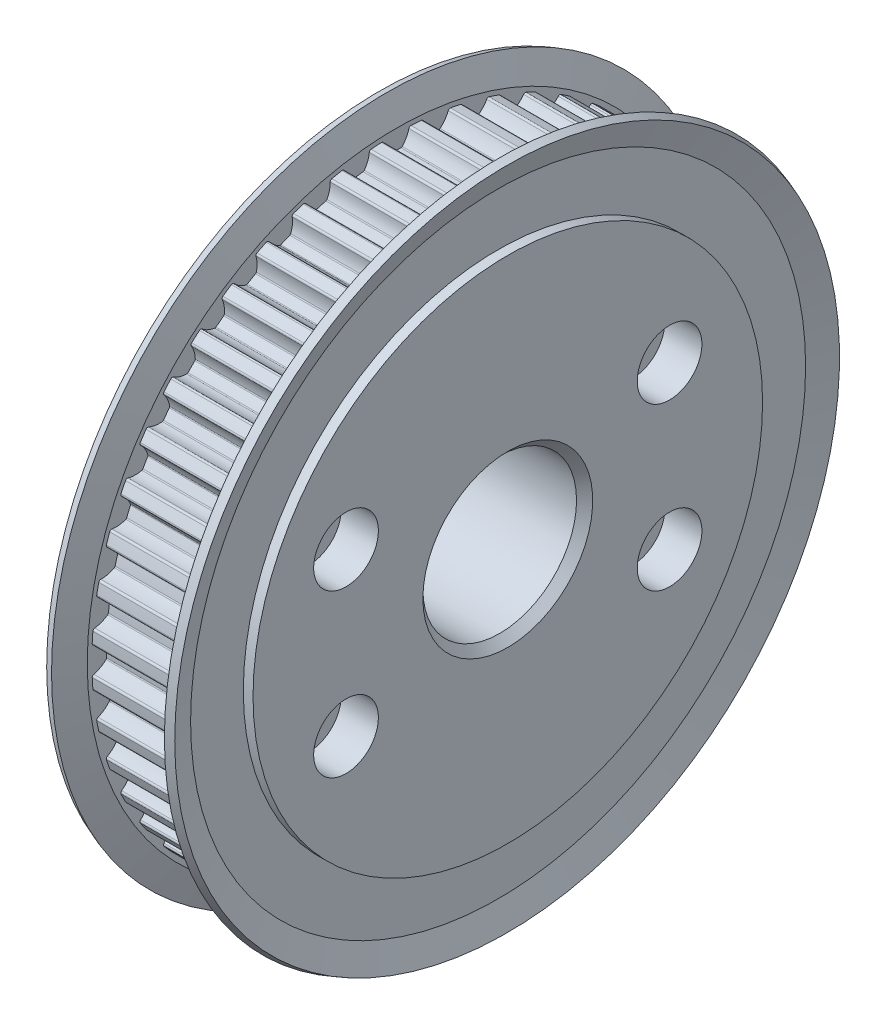
from build123d import *

# Parameters (mm, degrees)
SKETCH2_W                                            = 12
SKETCH2_H                                            = 30
SKETCH3_W                                            = 152.78
SKETCH3_H                                            = 152.78
CUT_EXTRUDE1_DEPTH                                   = 11.6
SKETCH4_R                                            = 9.5
CUT_EXTRUDE2_DEPTH                                   = 61.744199967
HOLE_SIZE_BY_SOCKET_HEAD_CAP_SCREW_TYPE1_D           = 4.5
HOLE_SIZE_BY_SOCKET_HEAD_CAP_SCREW_TYPE1_CBORE_D     = 8
HOLE_SIZE_BY_SOCKET_HEAD_CAP_SCREW_TYPE1_CBORE_DEPTH = 4.6
CHAMFER1_SIZE                                        = 1


with BuildPart() as part:
    # Sketch1 → Revolve1 (revolve)
    with BuildSketch(Plane.XY, mode=Mode.PRIVATE) as revolve1_sk:
        Polygon((0, 31.5), (0, 7.7), (0.2, 7.5), (27.8, 7.5), (28, 7.7), (28, 28.8), (27.8, 29), (16, 29), (16, 31.5), (14.8, 31.5), (14.8, 38.019075537), (15.916664119, 41.094554632), (14.97670473, 41.435840945), (13.8, 38.195), (2.2, 38.195), (1.02329527, 41.435840945), (0.083335881, 41.094554632), (1.2, 38.019075537), (1.2, 31.5), align=None)
    revolve(revolve1_sk.sketch.rotate(Axis((28, 0, 0), (-1, 0, 0)), 270), axis=Axis((28, 0, 0), (-1, 0, 0)))

    # Sketch2 → Cut-Revolve1 (revolve, cut)
    with BuildSketch(Plane.XY, mode=Mode.PRIVATE) as cut_revolve1_sk:
        with Locations((22, 15)):
            Rectangle(SKETCH2_W, SKETCH2_H)
    revolve(cut_revolve1_sk.sketch.rotate(Axis((28, 0, 0), (-1, 0, 0)), 270), axis=Axis((28, 0, 0), (-1, 0, 0)), mode=Mode.SUBTRACT)

    # Sketch3 → Cut-Extrude1 (cut)
    with BuildSketch(Plane(origin=(2.2, 0, 0), x_dir=(0, 0, -1), z_dir=(1, 0, 0))):
        Rectangle(SKETCH3_W, SKETCH3_H)
        with BuildLine():
            ThreePointArc((-37.580722706, 1.824802974), (-37.530923747, 1.662553905), (-37.388992694, 1.569493317))
            ThreePointArc((-37.388992694, 1.569493317), (-36.576235091, 1.258482416), (-35.87221643, 0.746954873))
            ThreePointArc((-35.87221643, 0.746954873), (-35.825535624, 0.679315888), (-35.809997004, 0.598614703))
            ThreePointArc((-35.809997004, 0.598614703), (-35.815, -3.6e-08), (-35.809997003, -0.598614776))
            ThreePointArc((-35.809997003, -0.598614776), (-35.825535638, -0.679315922), (-35.87221643, -0.746954873))
            ThreePointArc((-35.87221643, -0.746954873), (-36.57623506, -1.258482399), (-37.388992626, -1.569493301))
            ThreePointArc((-37.388992626, -1.569493301), (-37.530923726, -1.662553877), (-37.580722706, -1.824802974))
            ThreePointArc((-37.580722706, -1.824802974), (-37.563928353, -2.14287464), (-37.544441987, -2.460792737))
            ThreePointArc((-37.544441987, -2.460792737), (-37.522265005, -2.778534482), (-37.497398997, -3.096077104))
            ThreePointArc((-37.497398997, -3.096077104), (-37.426848324, -3.25043804), (-37.273984668, -3.324176762))
            ThreePointArc((-37.273984668, -3.324176762), (-36.427585249, -3.526440767), (-35.662821821, -3.941699246))
            ThreePointArc((-35.662821821, -3.941699246), (-35.607711717, -4.002666503), (-35.581772413, -4.080649081))
            ThreePointArc((-35.581772413, -4.080649081), (-35.508597705, -4.67479561), (-35.425502607, -5.267636096))
            ThreePointArc((-35.425502607, -5.267636096), (-35.430374694, -5.349675031), (-35.467827471, -5.422828388))
            ThreePointArc((-35.467827471, -5.422828388), (-36.099055384, -6.021872596), (-36.864264626, -6.436308907))
            ThreePointArc((-36.864264626, -6.436308907), (-36.992834644, -6.547099062), (-37.02102983, -6.714460168))
            ThreePointArc((-37.02102983, -6.714460168), (-36.962862471, -7.027618583), (-36.902046175, -7.340273366))
            ThreePointArc((-36.902046175, -7.340273366), (-36.838585301, -7.652402109), (-36.772484396, -7.963982444))
            ThreePointArc((-36.772484396, -7.963982444), (-36.682389148, -8.10781409), (-36.521208429, -8.160969257))
            ThreePointArc((-36.521208429, -8.160969257), (-35.655649323, -8.251025572), (-34.843226443, -8.562909799))
            ThreePointArc((-34.843226443, -8.562909799), (-34.78062999, -8.61616216), (-34.744733831, -8.690091828))
            ThreePointArc((-34.744733831, -8.690091828), (-34.594633459, -9.269604136), (-34.43486804, -9.846526701))
            ThreePointArc((-34.43486804, -9.846526701), (-34.428990216, -9.928499717), (-34.456574149, -10.005915805))
            ThreePointArc((-34.456574149, -10.005915805), (-35.004210861, -10.682226883), (-35.708778839, -11.192997482))
            ThreePointArc((-35.708778839, -11.192997482), (-35.821787905, -11.319621568), (-35.827896869, -11.489231086))
            ThreePointArc((-35.827896869, -11.489231086), (-35.729351764, -11.792118024), (-35.628246122, -12.094159882))
            ThreePointArc((-35.628246122, -12.094159882), (-35.524587188, -12.395335014), (-35.418382391, -12.695621837))
            ThreePointArc((-35.418382391, -12.695621837), (-35.310284058, -12.826463233), (-35.143544035, -12.858125281))
            ThreePointArc((-35.143544035, -12.858125281), (-34.273635274, -12.83443305), (-33.427453801, -13.037606591))
            ThreePointArc((-33.427453801, -13.037606591), (-33.35844204, -13.082232894), (-33.313203221, -13.150844695))
            ThreePointArc((-33.313203221, -13.150844695), (-33.088745443, -13.705807164), (-32.855043333, -14.256940505))
            ThreePointArc((-32.855043333, -14.256940505), (-32.838516169, -14.337445021), (-32.855759291, -14.417799229))
            ThreePointArc((-32.855759291, -14.417799229), (-33.310434585, -15.159805306), (-33.942305944, -15.758170768))
            ThreePointArc((-33.942305944, -15.758170768), (-34.037820443, -15.89846221), (-34.021738659, -16.067418075))
            ThreePointArc((-34.021738659, -16.067418075), (-33.884501943, -16.354851056), (-33.7448369, -16.641111969))
            ThreePointArc((-33.7448369, -16.641111969), (-33.602753539, -16.926180301), (-33.458262043, -17.21003562))
            ThreePointArc((-33.458262043, -17.21003562), (-33.334010276, -17.325647987), (-33.164564009, -17.33527522))
            ThreePointArc((-33.164564009, -17.33527522), (-32.305189896, -17.198239802), (-31.439728155, -17.289226319))
            ThreePointArc((-31.439728155, -17.289226319), (-31.365481893, -17.324463001), (-31.311674459, -17.386582976))
            ThreePointArc((-31.311674459, -17.386582976), (-31.016699814, -17.907500038), (-30.713059726, -18.423414104))
            ThreePointArc((-30.713059726, -18.423414104), (-30.686166006, -18.501072665), (-30.692773282, -18.582990111))
            ThreePointArc((-30.692773282, -18.582990111), (-31.046707538, -19.377995258), (-31.595070785, -20.053717383))
            ThreePointArc((-31.595070785, -20.053717383), (-31.671456436, -20.205275756), (-31.633459069, -20.370687086))
            ThreePointArc((-31.633459069, -20.370687086), (-31.459878899, -20.637748052), (-31.284044163, -20.903330017))
            ThreePointArc((-31.284044163, -20.903330017), (-31.105967461, -21.167413949), (-30.925661556, -21.429980923))
            ThreePointArc((-30.925661556, -21.429980923), (-30.787382335, -21.5283861), (-30.618129095, -21.515813792))
            ThreePointArc((-30.618129095, -21.515813792), (-29.783993761, -21.267779902), (-28.914060045, -21.245022592))
            ThreePointArc((-28.914060045, -21.245022592), (-28.835849659, -21.270266737), (-28.774394272, -21.324831987))
            ThreePointArc((-28.774394272, -21.324831987), (-28.413949856, -21.802790615), (-28.045567152, -22.27465798))
            ThreePointArc((-28.045567152, -22.27465798), (-28.008767035, -22.348141826), (-28.004625413, -22.43022088))
            ThreePointArc((-28.004625413, -22.43022088), (-28.251762717, -23.264622338), (-28.707235205, -24.006139333))
            ThreePointArc((-28.707235205, -24.006139333), (-28.763185029, -24.166371431), (-28.703922223, -24.325407993))
            ThreePointArc((-28.703922223, -24.325407993), (-28.496968605, -24.567527457), (-28.287972756, -24.807886293))
            ThreePointArc((-28.287972756, -24.807886293), (-28.076949655, -25.046467277), (-27.863914425, -25.28325331))
            ThreePointArc((-27.863914425, -25.28325331), (-27.713973748, -25.362767557), (-27.547809509, -25.328210825))
            ThreePointArc((-27.547809509, -25.328210825), (-26.753185238, -24.973422391), (-25.89366435, -24.837310638))
            ThreePointArc((-25.89366435, -24.837310638), (-25.812828043, -24.852130312), (-25.744776221, -24.898207211))
            ThreePointArc((-25.744776221, -24.898207211), (-25.325029337, -25.325029399), (-24.898207148, -25.744776282))
            ThreePointArc((-24.898207148, -25.744776282), (-24.852130295, -25.812828084), (-24.837310638, -25.89366435))
            ThreePointArc((-24.837310638, -25.89366435), (-24.973422403, -26.75318528), (-25.328210871, -27.547809584))
            ThreePointArc((-25.328210871, -27.547809584), (-25.362767551, -27.713973791), (-25.28325331, -27.863914425))
            ThreePointArc((-25.28325331, -27.863914425), (-25.046467277, -28.076949655), (-24.807886293, -28.287972756))
            ThreePointArc((-24.807886293, -28.287972756), (-24.567527457, -28.496968605), (-24.325407993, -28.703922223))
            ThreePointArc((-24.325407993, -28.703922223), (-24.166371472, -28.763185028), (-24.006139396, -28.707235256))
            ThreePointArc((-24.006139396, -28.707235256), (-23.264622375, -28.251762734), (-22.43022088, -28.004625413))
            ThreePointArc((-22.43022088, -28.004625413), (-22.348141783, -28.008767047), (-22.274657911, -28.045567207))
            ThreePointArc((-22.274657911, -28.045567207), (-21.802790545, -28.413949909), (-21.324831916, -28.774394325))
            ThreePointArc((-21.324831916, -28.774394325), (-21.270266715, -28.835849698), (-21.245022592, -28.914060045))
            ThreePointArc((-21.245022592, -28.914060045), (-21.267779908, -29.783993804), (-21.515813827, -30.618129175))
            ThreePointArc((-21.515813827, -30.618129175), (-21.528386088, -30.787382376), (-21.429980923, -30.925661556))
            ThreePointArc((-21.429980923, -30.925661556), (-21.167413949, -31.105967461), (-20.903330017, -31.284044163))
            ThreePointArc((-20.903330017, -31.284044163), (-20.637748052, -31.459878899), (-20.370687086, -31.633459069))
            ThreePointArc((-20.370687086, -31.633459069), (-20.205275801, -31.671456442), (-20.053717445, -31.595070851))
            ThreePointArc((-20.053717445, -31.595070851), (-19.377995297, -31.046707562), (-18.582990111, -30.692773282))
            ThreePointArc((-18.582990111, -30.692773282), (-18.501072611, -30.686166013), (-18.423414012, -30.713059781))
            ThreePointArc((-18.423414012, -30.713059781), (-17.907499953, -31.016699863), (-17.386582899, -31.311674502))
            ThreePointArc((-17.386582899, -31.311674502), (-17.324462974, -31.365481928), (-17.289226319, -31.439728155))
            ThreePointArc((-17.289226319, -31.439728155), (-17.198239803, -32.305189937), (-17.335275243, -33.164564086))
            ThreePointArc((-17.335275243, -33.164564086), (-17.325647971, -33.334010313), (-17.21003562, -33.458262043))
            ThreePointArc((-17.21003562, -33.458262043), (-16.926180301, -33.602753539), (-16.64111197, -33.7448369))
            ThreePointArc((-16.64111197, -33.7448369), (-16.354851056, -33.884501943), (-16.067418075, -34.021738659))
            ThreePointArc((-16.067418075, -34.021738659), (-15.898462259, -34.037820456), (-15.758170827, -33.942306026))
            ThreePointArc((-15.758170827, -33.942306026), (-15.159805346, -33.310434617), (-14.417799229, -32.855759291))
            ThreePointArc((-14.417799229, -32.855759291), (-14.337444967, -32.838516169), (-14.256940407, -32.855043376))
            ThreePointArc((-14.256940407, -32.855043376), (-13.70580708, -33.088745478), (-13.150844627, -33.313203247))
            ThreePointArc((-13.150844627, -33.313203247), (-13.082232868, -33.358442066), (-13.037606591, -33.427453801))
            ThreePointArc((-13.037606591, -33.427453801), (-12.834433046, -34.273635313), (-12.858125293, -35.143544112))
            ThreePointArc((-12.858125293, -35.143544112), (-12.826463213, -35.310284091), (-12.695621837, -35.418382391))
            ThreePointArc((-12.695621837, -35.418382391), (-12.395335014, -35.524587188), (-12.094159882, -35.628246122))
            ThreePointArc((-12.094159882, -35.628246122), (-11.792118024, -35.729351765), (-11.489231086, -35.827896869))
            ThreePointArc((-11.489231086, -35.827896869), (-11.319621613, -35.821787923), (-11.192997529, -35.708778924))
            ThreePointArc((-11.192997529, -35.708778924), (-10.682226916, -35.004210896), (-10.005915805, -34.456574149))
            ThreePointArc((-10.005915805, -34.456574149), (-9.928499664, -34.428990208), (-9.846526598, -34.434868069))
            ThreePointArc((-9.846526598, -34.434868069), (-9.269604048, -34.594633483), (-8.690091757, -34.744733849))
            ThreePointArc((-8.690091757, -34.744733849), (-8.616162131, -34.780630012), (-8.562909799, -34.843226443))
            ThreePointArc((-8.562909799, -34.843226443), (-8.251025581, -35.655649286), (-8.160969255, -36.521208354))
            ThreePointArc((-8.160969255, -36.521208354), (-8.107814114, -36.682389119), (-7.963982444, -36.772484396))
            ThreePointArc((-7.963982444, -36.772484396), (-7.652402109, -36.838585301), (-7.340273366, -36.902046175))
            ThreePointArc((-7.340273366, -36.902046175), (-7.027618583, -36.962862471), (-6.714460168, -37.02102983))
            ThreePointArc((-6.714460168, -37.02102983), (-6.547099105, -36.992834668), (-6.436308941, -36.864264717))
            ThreePointArc((-6.436308941, -36.864264717), (-6.021872624, -36.099055423), (-5.422828388, -35.467827471))
            ThreePointArc((-5.422828388, -35.467827471), (-5.349674979, -35.43037468), (-5.267635989, -35.425502623))
            ThreePointArc((-5.267635989, -35.425502623), (-4.674795521, -35.508597717), (-4.080649009, -35.581772422))
            ThreePointArc((-4.080649009, -35.581772422), (-4.002666471, -35.607711735), (-3.941699246, -35.662821821))
            ThreePointArc((-3.941699246, -35.662821821), (-3.526440781, -36.427585215), (-3.32417677, -37.273984595))
            ThreePointArc((-3.32417677, -37.273984595), (-3.250438067, -37.426848298), (-3.096077104, -37.497398997))
            ThreePointArc((-3.096077104, -37.497398997), (-2.778534482, -37.522265005), (-2.460792737, -37.544441987))
            ThreePointArc((-2.460792737, -37.544441987), (-2.14287464, -37.563928353), (-1.824802974, -37.580722706))
            ThreePointArc((-1.824802974, -37.580722706), (-1.662553917, -37.530923757), (-1.569493325, -37.388992724))
            ThreePointArc((-1.569493325, -37.388992724), (-1.258482423, -36.576235105), (-0.746954873, -35.87221643))
            ThreePointArc((-0.746954873, -35.87221643), (-0.679315872, -35.825535618), (-0.598614668, -35.809997005))
            ThreePointArc((-0.598614668, -35.809997005), (5.4e-08, -35.815), (0.598614776, -35.809997003))
            ThreePointArc((0.598614776, -35.809997003), (0.679315922, -35.825535638), (0.746954873, -35.87221643))
            ThreePointArc((0.746954873, -35.87221643), (1.258482399, -36.57623506), (1.569493301, -37.388992626))
            ThreePointArc((1.569493301, -37.388992626), (1.662553877, -37.530923726), (1.824802974, -37.580722706))
            ThreePointArc((1.824802974, -37.580722706), (2.14287464, -37.563928353), (2.460792737, -37.544441987))
            ThreePointArc((2.460792737, -37.544441987), (2.778534482, -37.522265005), (3.096077104, -37.497398997))
            ThreePointArc((3.096077104, -37.497398997), (3.250438031, -37.426848333), (3.32417676, -37.273984695))
            ThreePointArc((3.32417676, -37.273984695), (3.526440763, -36.427585262), (3.941699246, -35.662821821))
            ThreePointArc((3.941699246, -35.662821821), (4.00266651, -35.607711713), (4.080649097, -35.581772412))
            ThreePointArc((4.080649097, -35.581772412), (4.674795618, -35.508597704), (5.267636096, -35.425502607))
            ThreePointArc((5.267636096, -35.425502607), (5.349675031, -35.430374694), (5.422828388, -35.467827471))
            ThreePointArc((5.422828388, -35.467827471), (6.021872596, -36.099055384), (6.436308907, -36.864264626))
            ThreePointArc((6.436308907, -36.864264626), (6.547099062, -36.992834644), (6.714460168, -37.02102983))
            ThreePointArc((6.714460168, -37.02102983), (7.027618583, -36.962862471), (7.340273366, -36.902046175))
            ThreePointArc((7.340273366, -36.902046175), (7.652402109, -36.838585301), (7.963982444, -36.772484396))
            ThreePointArc((7.963982444, -36.772484396), (8.107814082, -36.682389159), (8.160969258, -36.521208456))
            ThreePointArc((8.160969258, -36.521208456), (8.251025569, -35.655649336), (8.562909799, -34.843226443))
            ThreePointArc((8.562909799, -34.843226443), (8.616162166, -34.780629985), (8.690091843, -34.744733828))
            ThreePointArc((8.690091843, -34.744733828), (9.269604143, -34.594633457), (9.846526701, -34.43486804))
            ThreePointArc((9.846526701, -34.43486804), (9.928499717, -34.428990216), (10.005915805, -34.456574149))
            ThreePointArc((10.005915805, -34.456574149), (10.682226883, -35.004210861), (11.192997482, -35.708778839))
            ThreePointArc((11.192997482, -35.708778839), (11.319621568, -35.821787905), (11.489231086, -35.827896869))
            ThreePointArc((11.489231086, -35.827896869), (11.792118024, -35.729351764), (12.094159882, -35.628246122))
            ThreePointArc((12.094159882, -35.628246122), (12.395335014, -35.524587188), (12.695621837, -35.418382391))
            ThreePointArc((12.695621837, -35.418382391), (12.826463239, -35.310284047), (12.858125277, -35.14354401))
            ThreePointArc((12.858125277, -35.14354401), (12.834433051, -34.273635262), (13.037606591, -33.427453801))
            ThreePointArc((13.037606591, -33.427453801), (13.082232906, -33.358442028), (13.150844727, -33.313203208))
            ThreePointArc((13.150844727, -33.313203208), (13.70580718, -33.088745436), (14.256940505, -32.855043333))
            ThreePointArc((14.256940505, -32.855043333), (14.337445021, -32.838516169), (14.417799229, -32.855759291))
            ThreePointArc((14.417799229, -32.855759291), (15.159805306, -33.310434585), (15.758170768, -33.942305944))
            ThreePointArc((15.758170768, -33.942305944), (15.89846221, -34.037820443), (16.067418075, -34.021738659))
            ThreePointArc((16.067418075, -34.021738659), (16.354851056, -33.884501943), (16.641111969, -33.7448369))
            ThreePointArc((16.641111969, -33.7448369), (16.926180301, -33.602753539), (17.21003562, -33.458262043))
            ThreePointArc((17.21003562, -33.458262043), (17.32564799, -33.334010268), (17.335275215, -33.164563993))
            ThreePointArc((17.335275215, -33.164563993), (17.198239801, -32.305189888), (17.289226319, -31.439728155))
            ThreePointArc((17.289226319, -31.439728155), (17.324463006, -31.365481885), (17.386582993, -31.31167445))
            ThreePointArc((17.386582993, -31.31167445), (17.907500047, -31.01669981), (18.423414104, -30.713059726))
            ThreePointArc((18.423414104, -30.713059726), (18.501072665, -30.686166006), (18.582990111, -30.692773282))
            ThreePointArc((18.582990111, -30.692773282), (19.377995258, -31.046707538), (20.053717383, -31.595070785))
            ThreePointArc((20.053717383, -31.595070785), (20.205275756, -31.671456436), (20.370687086, -31.633459069))
            ThreePointArc((20.370687086, -31.633459069), (20.637748052, -31.459878899), (20.903330017, -31.284044163))
            ThreePointArc((20.903330017, -31.284044163), (21.167413949, -31.105967461), (21.429980923, -30.925661556))
            ThreePointArc((21.429980923, -30.925661556), (21.528386102, -30.787382325), (21.515813784, -30.618129078))
            ThreePointArc((21.515813784, -30.618129078), (21.2677799, -29.783993752), (21.245022592, -28.914060045))
            ThreePointArc((21.245022592, -28.914060045), (21.270266741, -28.835849651), (21.324832003, -28.77439426))
            ThreePointArc((21.324832003, -28.77439426), (21.802790623, -28.41394985), (22.27465798, -28.045567152))
            ThreePointArc((22.27465798, -28.045567152), (22.348141826, -28.008767035), (22.43022088, -28.004625413))
            ThreePointArc((22.43022088, -28.004625413), (23.264622338, -28.251762717), (24.006139333, -28.707235205))
            ThreePointArc((24.006139333, -28.707235205), (24.166371431, -28.763185029), (24.325407993, -28.703922223))
            ThreePointArc((24.325407993, -28.703922223), (24.567527457, -28.496968605), (24.807886293, -28.287972756))
            ThreePointArc((24.807886293, -28.287972756), (25.046467277, -28.076949655), (25.28325331, -27.863914425))
            ThreePointArc((25.28325331, -27.863914425), (25.362767558, -27.713973738), (25.328210815, -27.547809492))
            ThreePointArc((25.328210815, -27.547809492), (24.973422388, -26.753185229), (24.837310638, -25.89366435))
            ThreePointArc((24.837310638, -25.89366435), (24.852130315, -25.812828034), (24.898207225, -25.744776208))
            ThreePointArc((24.898207225, -25.744776208), (25.325029406, -25.32502933), (25.744776282, -24.898207148))
            ThreePointArc((25.744776282, -24.898207148), (25.812828084, -24.852130295), (25.89366435, -24.837310638))
            ThreePointArc((25.89366435, -24.837310638), (26.75318528, -24.973422403), (27.547809584, -25.328210871))
            ThreePointArc((27.547809584, -25.328210871), (27.713973791, -25.362767551), (27.863914425, -25.28325331))
            ThreePointArc((27.863914425, -25.28325331), (28.076949655, -25.046467277), (28.287972756, -24.807886293))
            ThreePointArc((28.287972756, -24.807886293), (28.496968605, -24.567527457), (28.703922223, -24.325407993))
            ThreePointArc((28.703922223, -24.325407993), (28.763185029, -24.166371377), (28.707235137, -24.00613925))
            ThreePointArc((28.707235137, -24.00613925), (28.251762695, -23.264622289), (28.004625412, -22.43022088))
            ThreePointArc((28.004625412, -22.43022088), (28.00876705, -22.348141768), (28.045567226, -22.274657887))
            ThreePointArc((28.045567226, -22.274657887), (28.413949919, -21.802790533), (28.774394324, -21.324831916))
            ThreePointArc((28.774394324, -21.324831916), (28.835849698, -21.270266715), (28.914060045, -21.245022592))
            ThreePointArc((28.914060045, -21.245022592), (29.783993804, -21.267779908), (30.618129174, -21.515813827))
            ThreePointArc((30.618129174, -21.515813827), (30.787382376, -21.528386088), (30.925661556, -21.429980923))
            ThreePointArc((30.925661556, -21.429980923), (31.105967461, -21.167413949), (31.284044163, -20.903330017))
            ThreePointArc((31.284044163, -20.903330017), (31.459878899, -20.637748052), (31.633459069, -20.370687086))
            ThreePointArc((31.633459069, -20.370687086), (31.67145643, -20.205275701), (31.595070705, -20.053717307))
            ThreePointArc((31.595070705, -20.053717307), (31.046707509, -19.377995211), (30.692773282, -18.582990111))
            ThreePointArc((30.692773282, -18.582990111), (30.686166014, -18.501072606), (30.713059787, -18.423414003))
            ThreePointArc((30.713059787, -18.423414003), (31.016699866, -17.907499949), (31.311674502, -17.386582898))
            ThreePointArc((31.311674502, -17.386582898), (31.365481928, -17.324462974), (31.439728155, -17.289226319))
            ThreePointArc((31.439728155, -17.289226319), (32.305189937, -17.198239803), (33.164564086, -17.335275243))
            ThreePointArc((33.164564086, -17.335275243), (33.334010313, -17.325647971), (33.458262043, -17.21003562))
            ThreePointArc((33.458262043, -17.21003562), (33.602753539, -16.926180301), (33.7448369, -16.641111969))
            ThreePointArc((33.7448369, -16.641111969), (33.884501943, -16.354851056), (34.021738659, -16.067418075))
            ThreePointArc((34.021738659, -16.067418075), (34.03782043, -15.89846216), (33.942305861, -15.758170707))
            ThreePointArc((33.942305861, -15.758170707), (33.310434552, -15.159805266), (32.855759291, -14.417799229))
            ThreePointArc((32.855759291, -14.417799229), (32.838516169, -14.337444956), (32.855043385, -14.256940387))
            ThreePointArc((32.855043385, -14.256940387), (33.088745482, -13.705807071), (33.313203247, -13.150844627))
            ThreePointArc((33.313203247, -13.150844627), (33.358442066, -13.082232868), (33.427453801, -13.037606591))
            ThreePointArc((33.427453801, -13.037606591), (34.273635313, -12.834433046), (35.143544112, -12.858125293))
            ThreePointArc((35.143544112, -12.858125293), (35.310284091, -12.826463213), (35.418382391, -12.695621837))
            ThreePointArc((35.418382391, -12.695621837), (35.524587188, -12.395335014), (35.628246122, -12.094159882))
            ThreePointArc((35.628246122, -12.094159882), (35.729351764, -11.792118024), (35.827896869, -11.489231086))
            ThreePointArc((35.827896869, -11.489231086), (35.821787885, -11.319621519), (35.708778745, -11.192997432))
            ThreePointArc((35.708778745, -11.192997432), (35.004210822, -10.682226846), (34.456574149, -10.005915805))
            ThreePointArc((34.456574149, -10.005915805), (34.428990207, -9.928499653), (34.434868075, -9.846526577))
            ThreePointArc((34.434868075, -9.846526577), (34.594633485, -9.269604038), (34.744733849, -8.690091757))
            ThreePointArc((34.744733849, -8.690091757), (34.780630012, -8.616162131), (34.843226443, -8.562909799))
            ThreePointArc((34.843226443, -8.562909799), (35.655649286, -8.251025581), (36.521208354, -8.160969255))
            ThreePointArc((36.521208354, -8.160969255), (36.682389119, -8.107814114), (36.772484396, -7.963982444))
            ThreePointArc((36.772484396, -7.963982444), (36.838585301, -7.652402109), (36.902046175, -7.340273366))
            ThreePointArc((36.902046175, -7.340273366), (36.962862471, -7.027618583), (37.02102983, -6.714460168))
            ThreePointArc((37.02102983, -6.714460168), (36.992834618, -6.547099017), (36.864264528, -6.436308869))
            ThreePointArc((36.864264528, -6.436308869), (36.099055341, -6.021872565), (35.467827471, -5.422828388))
            ThreePointArc((35.467827471, -5.422828388), (35.430374677, -5.349674969), (35.425502626, -5.267635968))
            ThreePointArc((35.425502626, -5.267635968), (35.508597719, -4.67479551), (35.581772422, -4.080649009))
            ThreePointArc((35.581772422, -4.080649009), (35.607711735, -4.002666471), (35.662821821, -3.941699246))
            ThreePointArc((35.662821821, -3.941699246), (36.427585215, -3.526440781), (37.273984595, -3.32417677))
            ThreePointArc((37.273984595, -3.32417677), (37.426848298, -3.250438067), (37.497398997, -3.096077104))
            ThreePointArc((37.497398997, -3.096077104), (37.522265005, -2.778534482), (37.544441987, -2.460792737))
            ThreePointArc((37.544441987, -2.460792737), (37.563928353, -2.14287464), (37.580722706, -1.824802974))
            ThreePointArc((37.580722706, -1.824802974), (37.530923693, -1.662553832), (37.388992518, -1.569493275))
            ThreePointArc((37.388992518, -1.569493275), (36.576235012, -1.258482373), (35.87221643, -0.746954873))
            ThreePointArc((35.87221643, -0.746954873), (35.825535614, -0.679315862), (35.809997005, -0.598614647))
            ThreePointArc((35.809997005, -0.598614647), (35.815, 6.4e-08), (35.809997003, 0.598614776))
            ThreePointArc((35.809997003, 0.598614776), (35.825535638, 0.679315922), (35.87221643, 0.746954873))
            ThreePointArc((35.87221643, 0.746954873), (36.57623506, 1.258482399), (37.388992626, 1.569493301))
            ThreePointArc((37.388992626, 1.569493301), (37.530923726, 1.662553877), (37.580722706, 1.824802974))
            ThreePointArc((37.580722706, 1.824802974), (37.563928353, 2.14287464), (37.544441987, 2.460792737))
            ThreePointArc((37.544441987, 2.460792737), (37.522265005, 2.778534482), (37.497398997, 3.096077104))
            ThreePointArc((37.497398997, 3.096077104), (37.426848259, 3.250438106), (37.273984485, 3.324176781))
            ThreePointArc((37.273984485, 3.324176781), (36.427585163, 3.5264408), (35.662821821, 3.941699246))
            ThreePointArc((35.662821821, 3.941699246), (35.607711703, 4.002666527), (35.581772407, 4.080649137))
            ThreePointArc((35.581772407, 4.080649137), (35.508597702, 4.674795638), (35.425502607, 5.267636096))
            ThreePointArc((35.425502607, 5.267636096), (35.430374694, 5.349675031), (35.467827471, 5.422828388))
            ThreePointArc((35.467827471, 5.422828388), (36.099055384, 6.021872596), (36.864264626, 6.436308907))
            ThreePointArc((36.864264626, 6.436308907), (36.992834644, 6.547099062), (37.02102983, 6.714460168))
            ThreePointArc((37.02102983, 6.714460168), (36.962862471, 7.027618583), (36.902046175, 7.340273366))
            ThreePointArc((36.902046175, 7.340273366), (36.838585301, 7.652402109), (36.772484396, 7.963982444))
            ThreePointArc((36.772484396, 7.963982444), (36.682389074, 8.107814148), (36.521208241, 8.160969252))
            ThreePointArc((36.521208241, 8.160969252), (35.655649232, 8.251025594), (34.843226443, 8.562909799))
            ThreePointArc((34.843226443, 8.562909799), (34.780629972, 8.616162182), (34.744733818, 8.690091882))
            ThreePointArc((34.744733818, 8.690091882), (34.594633452, 9.269604163), (34.43486804, 9.846526701))
            ThreePointArc((34.43486804, 9.846526701), (34.428990216, 9.928499717), (34.456574149, 10.005915805))
            ThreePointArc((34.456574149, 10.005915805), (35.004210861, 10.682226883), (35.708778839, 11.192997482))
            ThreePointArc((35.708778839, 11.192997482), (35.821787905, 11.319621568), (35.827896869, 11.489231086))
            ThreePointArc((35.827896869, 11.489231086), (35.729351764, 11.792118024), (35.628246122, 12.094159882))
            ThreePointArc((35.628246122, 12.094159882), (35.524587188, 12.395335014), (35.418382391, 12.695621837))
            ThreePointArc((35.418382391, 12.695621837), (35.310284041, 12.826463242), (35.143543997, 12.858125275))
            ThreePointArc((35.143543997, 12.858125275), (34.273635255, 12.834433052), (33.427453801, 13.037606591))
            ThreePointArc((33.427453801, 13.037606591), (33.35844202, 13.082232914), (33.3132032, 13.150844747))
            ThreePointArc((33.3132032, 13.150844747), (33.088745432, 13.70580719), (32.855043333, 14.256940505))
            ThreePointArc((32.855043333, 14.256940505), (32.838516169, 14.337445021), (32.855759291, 14.417799229))
            ThreePointArc((32.855759291, 14.417799229), (33.310434585, 15.159805306), (33.942305944, 15.758170768))
            ThreePointArc((33.942305944, 15.758170768), (34.037820443, 15.89846221), (34.021738659, 16.067418075))
            ThreePointArc((34.021738659, 16.067418075), (33.884501943, 16.354851056), (33.7448369, 16.641111969))
            ThreePointArc((33.7448369, 16.641111969), (33.602753539, 16.926180301), (33.458262043, 17.21003562))
            ThreePointArc((33.458262043, 17.21003562), (33.334010263, 17.325647992), (33.164563982, 17.335275212))
            ThreePointArc((33.164563982, 17.335275212), (32.305189882, 17.198239801), (31.439728155, 17.289226319))
            ThreePointArc((31.439728155, 17.289226319), (31.365481877, 17.324463013), (31.311674439, 17.386583011))
            ThreePointArc((31.311674439, 17.386583011), (31.016699804, 17.907500056), (30.713059726, 18.423414104))
            ThreePointArc((30.713059726, 18.423414104), (30.686166006, 18.501072665), (30.692773282, 18.582990111))
            ThreePointArc((30.692773282, 18.582990111), (31.046707538, 19.377995258), (31.595070785, 20.053717383))
            ThreePointArc((31.595070785, 20.053717383), (31.671456436, 20.205275756), (31.633459069, 20.370687086))
            ThreePointArc((31.633459069, 20.370687086), (31.459878899, 20.637748052), (31.284044163, 20.903330017))
            ThreePointArc((31.284044163, 20.903330017), (31.105967461, 21.167413949), (30.925661556, 21.429980923))
            ThreePointArc((30.925661556, 21.429980923), (30.787382325, 21.528386103), (30.618129077, 21.515813783))
            ThreePointArc((30.618129077, 21.515813783), (29.783993751, 21.2677799), (28.914060045, 21.245022592))
            ThreePointArc((28.914060045, 21.245022592), (28.835849642, 21.270266747), (28.774394248, 21.32483202))
            ThreePointArc((28.774394248, 21.32483202), (28.413949843, 21.802790631), (28.045567152, 22.27465798))
            ThreePointArc((28.045567152, 22.27465798), (28.008767035, 22.348141826), (28.004625412, 22.43022088))
            ThreePointArc((28.004625412, 22.43022088), (28.251762717, 23.264622338), (28.707235205, 24.006139333))
            ThreePointArc((28.707235205, 24.006139333), (28.763185029, 24.166371431), (28.703922223, 24.325407993))
            ThreePointArc((28.703922223, 24.325407993), (28.496968605, 24.567527457), (28.287972756, 24.807886293))
            ThreePointArc((28.287972756, 24.807886293), (28.076949655, 25.046467277), (27.863914425, 25.28325331))
            ThreePointArc((27.863914425, 25.28325331), (27.713973734, 25.362767559), (27.547809485, 25.328210811))
            ThreePointArc((27.547809485, 25.328210811), (26.753185225, 24.973422387), (25.89366435, 24.837310638))
            ThreePointArc((25.89366435, 24.837310638), (25.81282802, 24.852130321), (25.744776186, 24.898207247))
            ThreePointArc((25.744776186, 24.898207247), (25.325029319, 25.325029417), (24.898207148, 25.744776282))
            ThreePointArc((24.898207148, 25.744776282), (24.852130295, 25.812828084), (24.837310638, 25.89366435))
            ThreePointArc((24.837310638, 25.89366435), (24.973422403, 26.75318528), (25.328210871, 27.547809584))
            ThreePointArc((25.328210871, 27.547809584), (25.362767551, 27.713973791), (25.28325331, 27.863914425))
            ThreePointArc((25.28325331, 27.863914425), (25.046467277, 28.076949655), (24.807886293, 28.287972756))
            ThreePointArc((24.807886293, 28.287972756), (24.567527457, 28.496968605), (24.325407993, 28.703922223))
            ThreePointArc((24.325407993, 28.703922223), (24.166371372, 28.763185029), (24.00613924, 28.70723513))
            ThreePointArc((24.00613924, 28.70723513), (23.264622284, 28.251762693), (22.43022088, 28.004625413))
            ThreePointArc((22.43022088, 28.004625413), (22.348141759, 28.008767053), (22.274657872, 28.045567238))
            ThreePointArc((22.274657872, 28.045567238), (21.802790525, 28.413949925), (21.324831916, 28.774394324))
            ThreePointArc((21.324831916, 28.774394324), (21.270266715, 28.835849698), (21.245022592, 28.914060045))
            ThreePointArc((21.245022592, 28.914060045), (21.267779908, 29.783993804), (21.515813827, 30.618129174))
            ThreePointArc((21.515813827, 30.618129174), (21.528386088, 30.787382376), (21.429980923, 30.925661556))
            ThreePointArc((21.429980923, 30.925661556), (21.167413949, 31.105967461), (20.903330017, 31.284044163))
            ThreePointArc((20.903330017, 31.284044163), (20.637748052, 31.459878899), (20.370687086, 31.633459069))
            ThreePointArc((20.370687086, 31.633459069), (20.205275692, 31.671456428), (20.053717295, 31.595070692))
            ThreePointArc((20.053717295, 31.595070692), (19.377995204, 31.046707504), (18.582990111, 30.692773282))
            ThreePointArc((18.582990111, 30.692773282), (18.501072589, 30.686166016), (18.423413975, 30.713059804))
            ThreePointArc((18.423413975, 30.713059804), (17.907499934, 31.016699874), (17.386582898, 31.311674502))
            ThreePointArc((17.386582898, 31.311674502), (17.324462974, 31.365481928), (17.289226319, 31.439728155))
            ThreePointArc((17.289226319, 31.439728155), (17.198239802, 32.305189907), (17.335275226, 33.164564029))
            ThreePointArc((17.335275226, 33.164564029), (17.325647982, 33.334010285), (17.21003562, 33.458262043))
            ThreePointArc((17.21003562, 33.458262043), (16.926180301, 33.602753539), (16.641111969, 33.7448369))
            ThreePointArc((16.641111969, 33.7448369), (16.354851056, 33.884501943), (16.067418075, 34.021738659))
            ThreePointArc((16.067418075, 34.021738659), (15.898462149, 34.037820427), (15.758170694, 33.942305842))
            ThreePointArc((15.758170694, 33.942305842), (15.159805257, 33.310434545), (14.417799229, 32.855759291))
            ThreePointArc((14.417799229, 32.855759291), (14.337444945, 32.838516169), (14.256940367, 32.855043393))
            ThreePointArc((14.256940367, 32.855043393), (13.70580706, 33.088745486), (13.150844627, 33.313203247))
            ThreePointArc((13.150844627, 33.313203247), (13.082232868, 33.358442066), (13.037606591, 33.427453801))
            ThreePointArc((13.037606591, 33.427453801), (12.83443305, 34.273635271), (12.85812528, 35.143544028))
            ThreePointArc((12.85812528, 35.143544028), (12.826463234, 35.310284055), (12.695621837, 35.418382391))
            ThreePointArc((12.695621837, 35.418382391), (12.395335014, 35.524587188), (12.094159882, 35.628246122))
            ThreePointArc((12.094159882, 35.628246122), (11.792118024, 35.729351764), (11.489231086, 35.827896869))
            ThreePointArc((11.489231086, 35.827896869), (11.319621507, 35.821787881), (11.19299742, 35.708778724))
            ThreePointArc((11.19299742, 35.708778724), (10.682226838, 35.004210813), (10.005915805, 34.456574149))
            ThreePointArc((10.005915805, 34.456574149), (9.928499642, 34.428990205), (9.846526556, 34.434868081))
            ThreePointArc((9.846526556, 34.434868081), (9.269604027, 34.594633488), (8.690091757, 34.744733849))
            ThreePointArc((8.690091757, 34.744733849), (8.616162131, 34.780630012), (8.562909799, 34.843226443))
            ThreePointArc((8.562909799, 34.843226443), (8.251025571, 35.655649327), (8.160969257, 36.521208438))
            ThreePointArc((8.160969257, 36.521208438), (8.107814088, 36.682389152), (7.963982444, 36.772484396))
            ThreePointArc((7.963982444, 36.772484396), (7.652402109, 36.838585301), (7.340273366, 36.902046175))
            ThreePointArc((7.340273366, 36.902046175), (7.027618583, 36.962862471), (6.714460168, 37.02102983))
            ThreePointArc((6.714460168, 37.02102983), (6.547099005, 36.992834612), (6.43630886, 36.864264504))
            ThreePointArc((6.43630886, 36.864264504), (6.021872557, 36.099055331), (5.422828388, 35.467827471))
            ThreePointArc((5.422828388, 35.467827471), (5.349674958, 35.430374674), (5.267635946, 35.425502629))
            ThreePointArc((5.267635946, 35.425502629), (4.674795499, 35.50859772), (4.080649009, 35.581772422))
            ThreePointArc((4.080649009, 35.581772422), (4.002666471, 35.607711735), (3.941699246, 35.662821821))
            ThreePointArc((3.941699246, 35.662821821), (3.526440766, 36.427585254), (3.324176761, 37.273984679))
            ThreePointArc((3.324176761, 37.273984679), (3.250438037, 37.426848327), (3.096077104, 37.497398997))
            ThreePointArc((3.096077104, 37.497398997), (2.778534482, 37.522265005), (2.460792737, 37.544441987))
            ThreePointArc((2.460792737, 37.544441987), (2.14287464, 37.563928353), (1.824802974, 37.580722706))
            ThreePointArc((1.824802974, 37.580722706), (1.662553877, 37.530923726), (1.569493301, 37.388992626))
            ThreePointArc((1.569493301, 37.388992626), (1.258482399, 36.57623506), (0.746954873, 35.87221643))
            ThreePointArc((0.746954873, 35.87221643), (0.679315914, 35.825535635), (0.598614759, 35.809997003))
            ThreePointArc((0.598614759, 35.809997003), (-9e-09, 35.815), (-0.598614776, 35.809997003))
            ThreePointArc((-0.598614776, 35.809997003), (-0.679315922, 35.825535638), (-0.746954873, 35.87221643))
            ThreePointArc((-0.746954873, 35.87221643), (-1.258482399, 36.576235061), (-1.569493301, 37.388992626))
            ThreePointArc((-1.569493301, 37.388992626), (-1.662553877, 37.530923726), (-1.824802974, 37.580722706))
            ThreePointArc((-1.824802974, 37.580722706), (-2.14287464, 37.563928353), (-2.460792737, 37.544441987))
            ThreePointArc((-2.460792737, 37.544441987), (-2.778534482, 37.522265005), (-3.096077104, 37.497398997))
            ThreePointArc((-3.096077104, 37.497398997), (-3.250438074, 37.426848291), (-3.324176772, 37.273984574))
            ThreePointArc((-3.324176772, 37.273984574), (-3.526440784, 36.427585205), (-3.941699246, 35.662821821))
            ThreePointArc((-3.941699246, 35.662821821), (-4.002666479, 35.607711731), (-4.080649026, 35.58177242))
            ThreePointArc((-4.080649026, 35.58177242), (-4.674795583, 35.508597709), (-5.267636096, 35.425502607))
            ThreePointArc((-5.267636096, 35.425502607), (-5.349675031, 35.430374694), (-5.422828388, 35.467827471))
            ThreePointArc((-5.422828388, 35.467827471), (-6.021872596, 36.099055384), (-6.436308907, 36.864264626))
            ThreePointArc((-6.436308907, 36.864264626), (-6.547099062, 36.992834644), (-6.714460168, 37.02102983))
            ThreePointArc((-6.714460168, 37.02102983), (-7.027618583, 36.962862471), (-7.340273366, 36.902046175))
            ThreePointArc((-7.340273366, 36.902046175), (-7.652402109, 36.838585301), (-7.963982444, 36.772484396))
            ThreePointArc((-7.963982444, 36.772484396), (-8.107814122, 36.682389108), (-8.160969254, 36.521208328))
            ThreePointArc((-8.160969254, 36.521208328), (-8.251025584, 35.655649273), (-8.562909799, 34.843226443))
            ThreePointArc((-8.562909799, 34.843226443), (-8.61616211, 34.780630028), (-8.690091706, 34.744733862))
            ThreePointArc((-8.690091706, 34.744733862), (-9.269604075, 34.594633475), (-9.846526701, 34.43486804))
            ThreePointArc((-9.846526701, 34.43486804), (-9.928499717, 34.428990216), (-10.005915805, 34.456574149))
            ThreePointArc((-10.005915805, 34.456574149), (-10.682226883, 35.004210861), (-11.192997482, 35.708778839))
            ThreePointArc((-11.192997482, 35.708778839), (-11.319621568, 35.821787905), (-11.489231086, 35.827896869))
            ThreePointArc((-11.489231086, 35.827896869), (-11.792118024, 35.729351765), (-12.094159882, 35.628246122))
            ThreePointArc((-12.094159882, 35.628246122), (-12.395335014, 35.524587188), (-12.695621837, 35.418382391))
            ThreePointArc((-12.695621837, 35.418382391), (-12.826463213, 35.310284091), (-12.858125293, 35.143544112))
            ThreePointArc((-12.858125293, 35.143544112), (-12.834433046, 34.273635313), (-13.037606591, 33.427453801))
            ThreePointArc((-13.037606591, 33.427453801), (-13.082232887, 33.358442047), (-13.150844676, 33.313203228))
            ThreePointArc((-13.150844676, 33.313203228), (-13.705807155, 33.088745447), (-14.256940505, 32.855043333))
            ThreePointArc((-14.256940505, 32.855043333), (-14.337445021, 32.838516169), (-14.417799229, 32.855759291))
            ThreePointArc((-14.417799229, 32.855759291), (-15.159805306, 33.310434585), (-15.758170768, 33.942305945))
            ThreePointArc((-15.758170768, 33.942305945), (-15.89846221, 34.037820443), (-16.067418075, 34.021738659))
            ThreePointArc((-16.067418075, 34.021738659), (-16.354851056, 33.884501943), (-16.64111197, 33.7448369))
            ThreePointArc((-16.64111197, 33.7448369), (-16.926180301, 33.602753539), (-17.21003562, 33.458262043))
            ThreePointArc((-17.21003562, 33.458262043), (-17.325647979, 33.334010294), (-17.335275231, 33.164564047))
            ThreePointArc((-17.335275231, 33.164564047), (-17.198239802, 32.305189916), (-17.289226319, 31.439728155))
            ThreePointArc((-17.289226319, 31.439728155), (-17.324462996, 31.365481899), (-17.386582962, 31.311674467))
            ThreePointArc((-17.386582962, 31.311674467), (-17.907500032, 31.016699818), (-18.423414104, 30.713059726))
            ThreePointArc((-18.423414104, 30.713059726), (-18.501072665, 30.686166006), (-18.582990111, 30.692773282))
            ThreePointArc((-18.582990111, 30.692773282), (-19.377995258, 31.046707538), (-20.053717383, 31.595070785))
            ThreePointArc((-20.053717383, 31.595070785), (-20.205275756, 31.671456436), (-20.370687086, 31.633459069))
            ThreePointArc((-20.370687086, 31.633459069), (-20.637748052, 31.459878899), (-20.903330017, 31.284044163))
            ThreePointArc((-20.903330017, 31.284044163), (-21.167413949, 31.105967461), (-21.429980923, 30.925661556))
            ThreePointArc((-21.429980923, 30.925661556), (-21.528386093, 30.787382358), (-21.515813811, 30.618129139))
            ThreePointArc((-21.515813811, 30.618129139), (-21.267779905, 29.783993785), (-21.245022592, 28.914060045))
            ThreePointArc((-21.245022592, 28.914060045), (-21.270266733, 28.835849666), (-21.324831975, 28.774394281))
            ThreePointArc((-21.324831975, 28.774394281), (-21.802790609, 28.41394986), (-22.27465798, 28.045567152))
            ThreePointArc((-22.27465798, 28.045567152), (-22.348141826, 28.008767035), (-22.43022088, 28.004625413))
            ThreePointArc((-22.43022088, 28.004625413), (-23.264622338, 28.251762717), (-24.006139333, 28.707235205))
            ThreePointArc((-24.006139333, 28.707235205), (-24.166371431, 28.763185029), (-24.325407993, 28.703922223))
            ThreePointArc((-24.325407993, 28.703922223), (-24.567527457, 28.496968605), (-24.807886293, 28.287972756))
            ThreePointArc((-24.807886293, 28.287972756), (-25.046467277, 28.076949655), (-25.28325331, 27.863914425))
            ThreePointArc((-25.28325331, 27.863914425), (-25.362767555, 27.713973762), (-25.32821084, 27.547809533))
            ThreePointArc((-25.32821084, 27.547809533), (-24.973422395, 26.753185251), (-24.837310638, 25.89366435))
            ThreePointArc((-24.837310638, 25.89366435), (-24.852130309, 25.812828051), (-24.8982072, 25.744776232))
            ThreePointArc((-24.8982072, 25.744776232), (-25.325029394, 25.325029342), (-25.744776282, 24.898207148))
            ThreePointArc((-25.744776282, 24.898207148), (-25.812828084, 24.852130295), (-25.89366435, 24.837310638))
            ThreePointArc((-25.89366435, 24.837310638), (-26.75318528, 24.973422403), (-27.547809584, 25.328210871))
            ThreePointArc((-27.547809584, 25.328210871), (-27.713973791, 25.362767551), (-27.863914425, 25.28325331))
            ThreePointArc((-27.863914425, 25.28325331), (-28.076949655, 25.046467277), (-28.287972756, 24.807886293))
            ThreePointArc((-28.287972756, 24.807886293), (-28.496968605, 24.567527457), (-28.703922223, 24.325407993))
            ThreePointArc((-28.703922223, 24.325407993), (-28.763185029, 24.166371405), (-28.707235172, 24.006139292))
            ThreePointArc((-28.707235172, 24.006139292), (-28.251762706, 23.264622314), (-28.004625413, 22.43022088))
            ThreePointArc((-28.004625413, 22.43022088), (-28.008767045, 22.348141791), (-28.045567197, 22.274657923))
            ThreePointArc((-28.045567197, 22.274657923), (-28.413949905, 21.802790551), (-28.774394324, 21.324831916))
            ThreePointArc((-28.774394324, 21.324831916), (-28.835849698, 21.270266715), (-28.914060045, 21.245022592))
            ThreePointArc((-28.914060045, 21.245022592), (-29.783993804, 21.267779908), (-30.618129175, 21.515813827))
            ThreePointArc((-30.618129175, 21.515813827), (-30.787382376, 21.528386088), (-30.925661556, 21.429980923))
            ThreePointArc((-30.925661556, 21.429980923), (-31.105967461, 21.167413949), (-31.284044163, 20.903330017))
            ThreePointArc((-31.284044163, 20.903330017), (-31.459878899, 20.637748052), (-31.633459069, 20.370687086))
            ThreePointArc((-31.633459069, 20.370687086), (-31.671456439, 20.205275782), (-31.595070823, 20.053717419))
            ThreePointArc((-31.595070823, 20.053717419), (-31.046707551, 19.37799528), (-30.692773282, 18.582990111))
            ThreePointArc((-30.692773282, 18.582990111), (-30.686166011, 18.501072628), (-30.713059764, 18.423414042))
            ThreePointArc((-30.713059764, 18.423414042), (-31.016699855, 17.907499968), (-31.311674502, 17.386582899))
            ThreePointArc((-31.311674502, 17.386582899), (-31.365481928, 17.324462974), (-31.439728155, 17.289226319))
            ThreePointArc((-31.439728155, 17.289226319), (-32.305189937, 17.198239803), (-33.164564086, 17.335275243))
            ThreePointArc((-33.164564086, 17.335275243), (-33.334010313, 17.325647971), (-33.458262043, 17.21003562))
            ThreePointArc((-33.458262043, 17.21003562), (-33.602753539, 16.926180301), (-33.7448369, 16.641111969))
            ThreePointArc((-33.7448369, 16.641111969), (-33.884501943, 16.354851056), (-34.021738659, 16.067418075))
            ThreePointArc((-34.021738659, 16.067418075), (-34.03782045, 15.898462239), (-33.942305993, 15.758170803))
            ThreePointArc((-33.942305993, 15.758170803), (-33.310434604, 15.15980533), (-32.855759291, 14.417799229))
            ThreePointArc((-32.855759291, 14.417799229), (-32.838516169, 14.337444984), (-32.855043362, 14.256940439))
            ThreePointArc((-32.855043362, 14.256940439), (-33.088745471, 13.705807097), (-33.313203247, 13.150844627))
            ThreePointArc((-33.313203247, 13.150844627), (-33.358442066, 13.082232868), (-33.427453801, 13.037606591))
            ThreePointArc((-33.427453801, 13.037606591), (-34.273635313, 12.834433046), (-35.143544112, 12.858125293))
            ThreePointArc((-35.143544112, 12.858125293), (-35.310284091, 12.826463213), (-35.418382391, 12.695621837))
            ThreePointArc((-35.418382391, 12.695621837), (-35.524587188, 12.395335014), (-35.628246122, 12.094159882))
            ThreePointArc((-35.628246122, 12.094159882), (-35.729351764, 11.792118024), (-35.827896869, 11.489231086))
            ThreePointArc((-35.827896869, 11.489231086), (-35.821787916, 11.319621596), (-35.708778891, 11.192997511))
            ThreePointArc((-35.708778891, 11.192997511), (-35.004210882, 10.682226903), (-34.456574149, 10.005915805))
            ThreePointArc((-34.456574149, 10.005915805), (-34.428990211, 9.928499681), (-34.43486806, 9.846526631))
            ThreePointArc((-34.43486806, 9.846526631), (-34.594633478, 9.269604065), (-34.744733849, 8.690091757))
            ThreePointArc((-34.744733849, 8.690091757), (-34.780630012, 8.616162131), (-34.843226443, 8.562909799))
            ThreePointArc((-34.843226443, 8.562909799), (-35.655649286, 8.251025581), (-36.521208354, 8.160969255))
            ThreePointArc((-36.521208354, 8.160969255), (-36.682389119, 8.107814114), (-36.772484396, 7.963982444))
            ThreePointArc((-36.772484396, 7.963982444), (-36.838585301, 7.652402109), (-36.902046175, 7.340273366))
            ThreePointArc((-36.902046175, 7.340273366), (-36.962862471, 7.027618583), (-37.02102983, 6.714460168))
            ThreePointArc((-37.02102983, 6.714460168), (-36.99283466, 6.547099091), (-36.864264688, 6.43630893))
            ThreePointArc((-36.864264688, 6.43630893), (-36.09905541, 6.021872615), (-35.467827471, 5.422828388))
            ThreePointArc((-35.467827471, 5.422828388), (-35.430374685, 5.349674996), (-35.425502618, 5.267636024))
            ThreePointArc((-35.425502618, 5.267636024), (-35.508597715, 4.674795538), (-35.581772422, 4.080649009))
            ThreePointArc((-35.581772422, 4.080649009), (-35.607711735, 4.002666471), (-35.662821821, 3.941699246))
            ThreePointArc((-35.662821821, 3.941699246), (-36.427585215, 3.526440781), (-37.273984595, 3.32417677))
            ThreePointArc((-37.273984595, 3.32417677), (-37.426848298, 3.250438067), (-37.497398997, 3.096077104))
            ThreePointArc((-37.497398997, 3.096077104), (-37.522265005, 2.778534482), (-37.544441987, 2.460792737))
            ThreePointArc((-37.544441987, 2.460792737), (-37.563928353, 2.14287464), (-37.580722706, 1.824802974))
        make_face(mode=Mode.SUBTRACT)
    extrude(amount=CUT_EXTRUDE1_DEPTH, mode=Mode.SUBTRACT)

    # Sketch4 → Cut-Extrude2 (cut, through all)
    with BuildSketch(Plane(origin=(16, 0, 0), x_dir=(0, 0, -1), z_dir=(1, 0, 0))):
        Circle(SKETCH4_R)
    extrude(amount=-CUT_EXTRUDE2_DEPTH, mode=Mode.SUBTRACT)

    # Hole size by socket head cap screw type1 (through all)
    with Locations(Plane(origin=(16, 0, 0), x_dir=(0, 0, -1), z_dir=(1, 0, 0))):
        with Locations((20, 10), (-20, 10), (-20, -10), (20, -10)):
            CounterBoreHole(HOLE_SIZE_BY_SOCKET_HEAD_CAP_SCREW_TYPE1_D / 2, HOLE_SIZE_BY_SOCKET_HEAD_CAP_SCREW_TYPE1_CBORE_D / 2, HOLE_SIZE_BY_SOCKET_HEAD_CAP_SCREW_TYPE1_CBORE_DEPTH)

    # Chamfer1
    chamfer1_edges = [part.edges().sort_by_distance(p)[0] for p in [
        (16, 0, 9.5),
        (0, 0, 9.5),
    ]]
    chamfer(chamfer1_edges, length=CHAMFER1_SIZE)


solid = part.part
